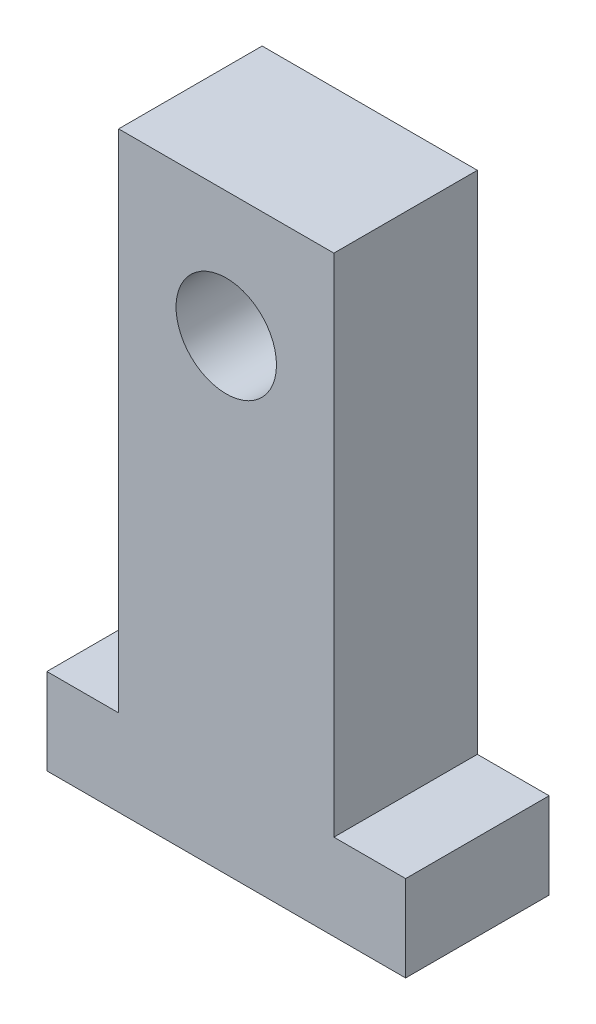
from build123d import *

# Parameters (mm, degrees)
SKETCH_1_W          = 50
SKETCH_1_H          = 82.5
EXTRUDE_1_DEPTH     = 20
SKETCH_2_R          = 7
CUT_EXTRUDE_1_DEPTH = 53.216496436
SKETCH_3_W          = 10
SKETCH_3_H          = 70.5
CUT_EXTRUDE_2_DEPTH = 53.216496436


with BuildPart() as part:
    # 草图1 → 凸台-拉伸1 (new body)
    with BuildSketch(Plane.XY):
        Rectangle(SKETCH_1_W, SKETCH_1_H)
    extrude(amount=EXTRUDE_1_DEPTH)

    # 草图2 → 切除-拉伸1 (cut, through all)
    with BuildSketch(Plane.XY.offset(20)):
        with Locations((0, 23.75)):
            Circle(SKETCH_2_R)
    extrude(amount=-CUT_EXTRUDE_1_DEPTH, mode=Mode.SUBTRACT)

    # 草图3 → 切除-拉伸2 (cut, through all)
    with BuildSketch(Plane.XY.offset(20)):
        with Locations((-20, 6)):
            Rectangle(SKETCH_3_W, SKETCH_3_H)
        with Locations((20, 6)):
            Rectangle(SKETCH_3_W, SKETCH_3_H)
    extrude(amount=-CUT_EXTRUDE_2_DEPTH, mode=Mode.SUBTRACT)


solid = part.part
